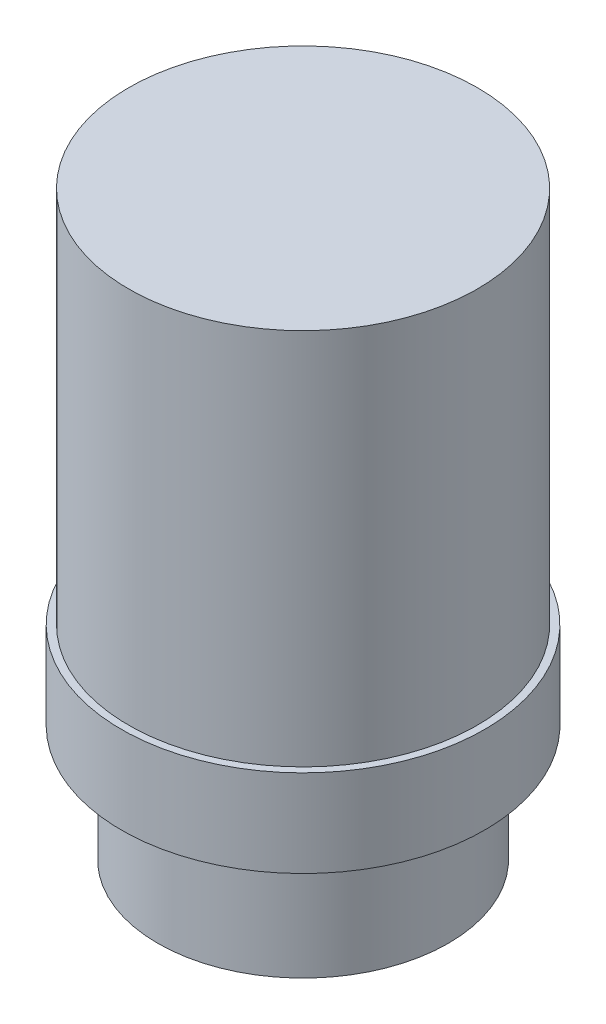
SolidWorks part; units mm, degrees
material "LY12#"
ref_plane "Front Plane" through (0, 0, 0) normal (0, 0, 1) x (1, 0, 0)
ref_plane "Top Plane" through (0, 0, 0) normal (0, 1, 0) x (1, 0, 0)
ref_plane "Right Plane" through (0, 0, 0) normal (1, 0, 0) x (0, 0, -1)
sketch "Sketch1" plane through (0, 0, 0) normal (0, 0, 1) x (1, 0, 0)
  line L0 (0, 0) -> (0, 40) construction
  line L1 (0, 40) -> (-12, 40)
  line L2 (-12, 40) -> (-12, 14)
  line L3 (-12, 14) -> (-12.5, 14)
  line L4 (-12.5, 14) -> (-12.5, 8)
  line L5 (-12.5, 8) -> (-10, 8)
  line L6 (-10, 8) -> (-10, 0)
  line L7 (-10, 0) -> (0, 0)
  line L8 (0, 0) -> (0, 40)
  dimension "D1" = 8
  dimension "D2" = 40
  dimension "D3" = 25
  dimension "D4" = 20
  dimension "D5" = 26
  dimension "D6" = 24
revolve "Revolve1" add sketch "Sketch1" angle 360 about L0
